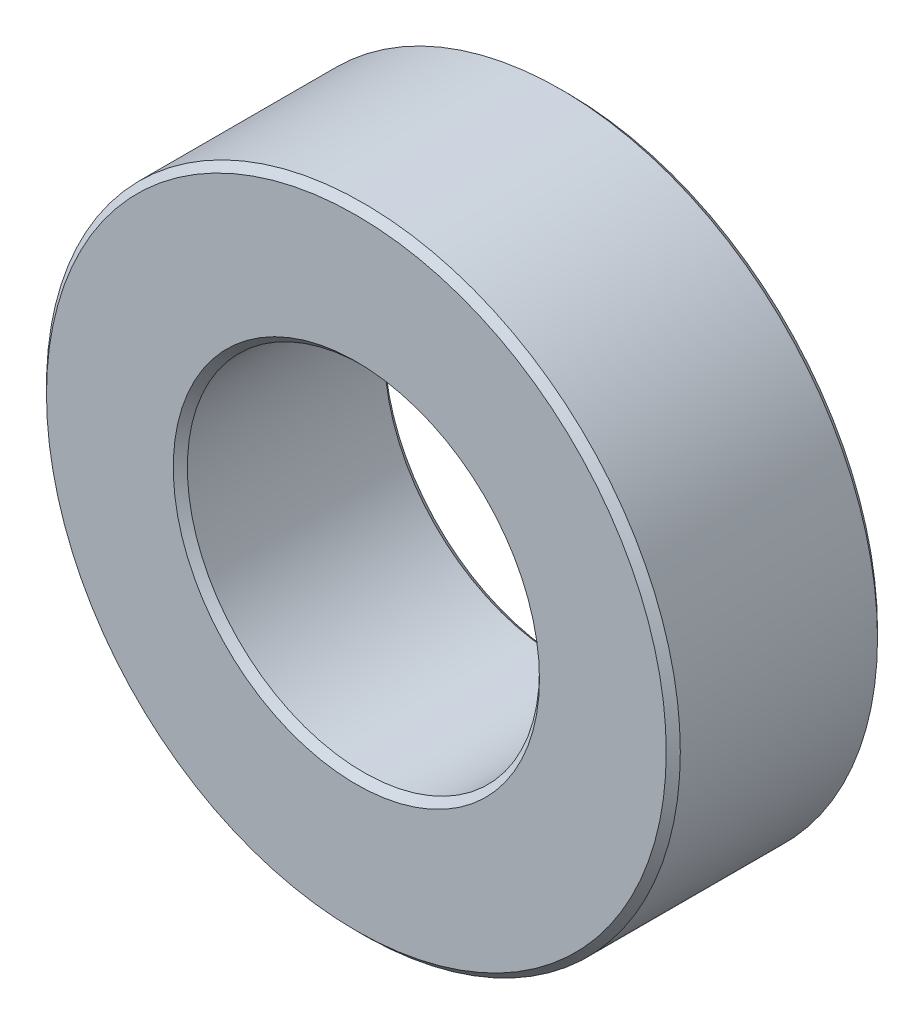
SolidWorks part; units mm, degrees
material "Q235"
ref_plane "Front Plane" through (0, 0, 0) normal (0, 0, 1) x (1, 0, 0)
ref_plane "Top Plane" through (0, 0, 0) normal (0, 1, 0) x (1, 0, 0)
ref_plane "Right Plane" through (0, 0, 0) normal (1, 0, 0) x (0, 0, -1)
sketch "Sketch1" plane through (0, 0, 0) normal (0, 0, 1) x (1, 0, 0)
  circle A0 centre (0, 0) radius 90
  circle A1 centre (0, 0) radius 50
  dimension "D1" = 180
  dimension "D2" = 100
extrude "Boss-Extrude1" add sketch "Sketch1" along normal blind 60
chamfer "Chamfer1" distance 2 angle 45 4 edges at (90, 0, 0) (50, 0, 0) (90, 0, 60) (50, 0, 60)
